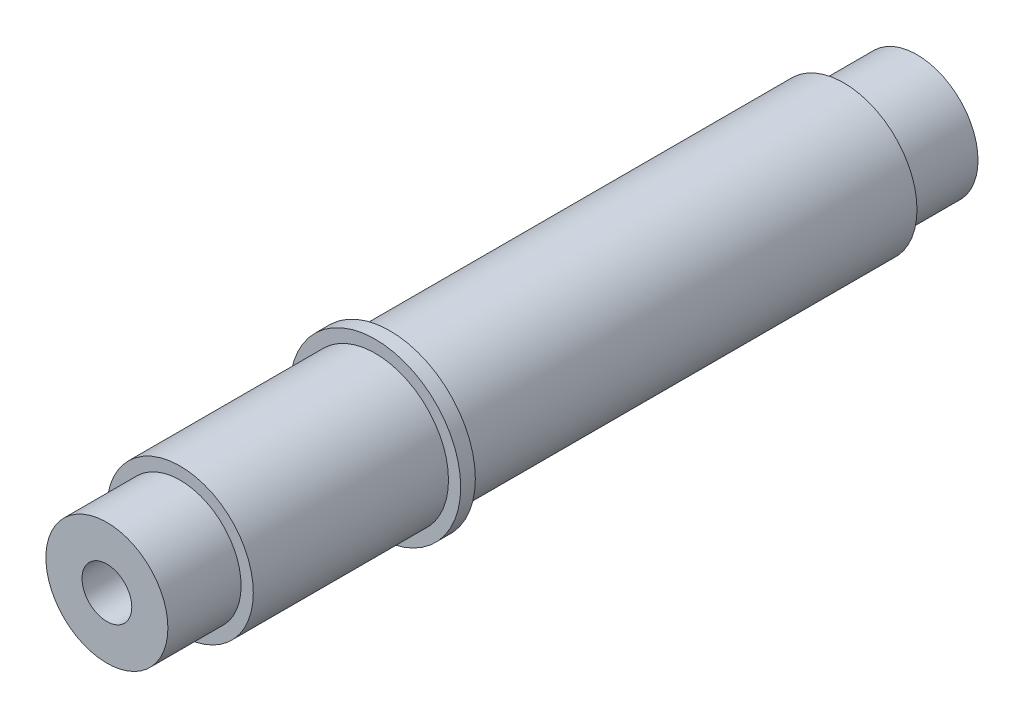
SolidWorks part; units mm, degrees
material "AISI 1045 钢，冷拔"
ref_plane "Front Plane" through (0, 0, 0) normal (0, 0, 1) x (1, 0, 0)
ref_plane "Top Plane" through (0, 0, 0) normal (0, 1, 0) x (1, 0, 0)
ref_plane "Right Plane" through (0, 0, 0) normal (1, 0, 0) x (0, 0, -1)
sketch "Sketch1" plane through (0, 0, 0) normal (0, 0, 1) x (1, 0, 0)
  circle A0 centre (0, 0) radius 15
  dimension "D1" = 30
extrude "Boss-Extrude1" add sketch "Sketch1" along normal mid plane 136
sketch "Sketch2" plane through (0, 0, 68) normal (0, 0, 1) x (1, 0, 0)
  circle A0 centre (0, 0) radius 12.5
  dimension "D1" = 25
extrude "Boss-Extrude2" add sketch "Sketch2" along normal blind 15
mirror "Mirror1" about plane through (0, 0, 0) normal (0, 0, 1) of "Boss-Extrude2"
sketch "Sketch4" plane through (0, 0, 0) normal (0, 0, 1) x (1, 0, 0)
  circle A0 centre (0, 0) radius 17.5
  dimension "D1" = 35
extrude "Boss-Extrude4" add sketch "Sketch4" along normal blind 3 from offset 25
hole_wizard "M12 Tapped Hole1" positions "Sketch6" profile "Sketch5" tap size "M12" standard "Iso"
sketch "Sketch6" plane through (0, 0, -83) normal (0, 0, -1) x (-1, 0, 0)
  point P0 (0, 0)
sketch "Sketch5" plane through (0, 0, -83) normal (1, 0, 0) x (0, 1, 0)
  line L0 (0, 0) -> (0, 35.8144)
  line L1 (0, 35.8144) -> (5.1, 32.75)
  line L2 (5.1, 32.75) -> (5.1, 0)
  line L5 (5.1, 0) -> (0, 0)
  line L10 (0, 35.8144) -> (-5.1, 32.75) construction
  line L11 (0, -6.35) -> (0, 107.95) construction
  dimension "螺纹孔钻头直径" = 10.2
  dimension "螺纹孔钻头深度" = 32.75
  dimension "导头角度" = 118
cosmetic thread "Cosmetic thread1" parameters "D1"=24, "D2"=12
hole_wizard "M12 Tapped Hole2" positions "Sketch8" profile "Sketch7" tap size "M12" standard "Iso"
sketch "Sketch8" plane through (0, 0, 83) normal (0, 0, 1) x (1, 0, 0)
  point P0 (0, 0)
sketch "Sketch7" plane through (0, 0, 83) normal (1, 0, 0) x (0, -1, 0)
  line L0 (0, 0) -> (0, 35.8144)
  line L1 (0, 35.8144) -> (5.1, 32.75)
  line L2 (5.1, 32.75) -> (5.1, 0)
  line L5 (5.1, 0) -> (0, 0)
  line L10 (0, 35.8144) -> (-5.1, 32.75) construction
  line L11 (0, -6.35) -> (0, 107.95) construction
  dimension "螺纹孔钻头直径" = 10.2
  dimension "螺纹孔钻头深度" = 32.75
  dimension "导头角度" = 118
cosmetic thread "Cosmetic thread2" parameters "D1"=24, "D2"=12
